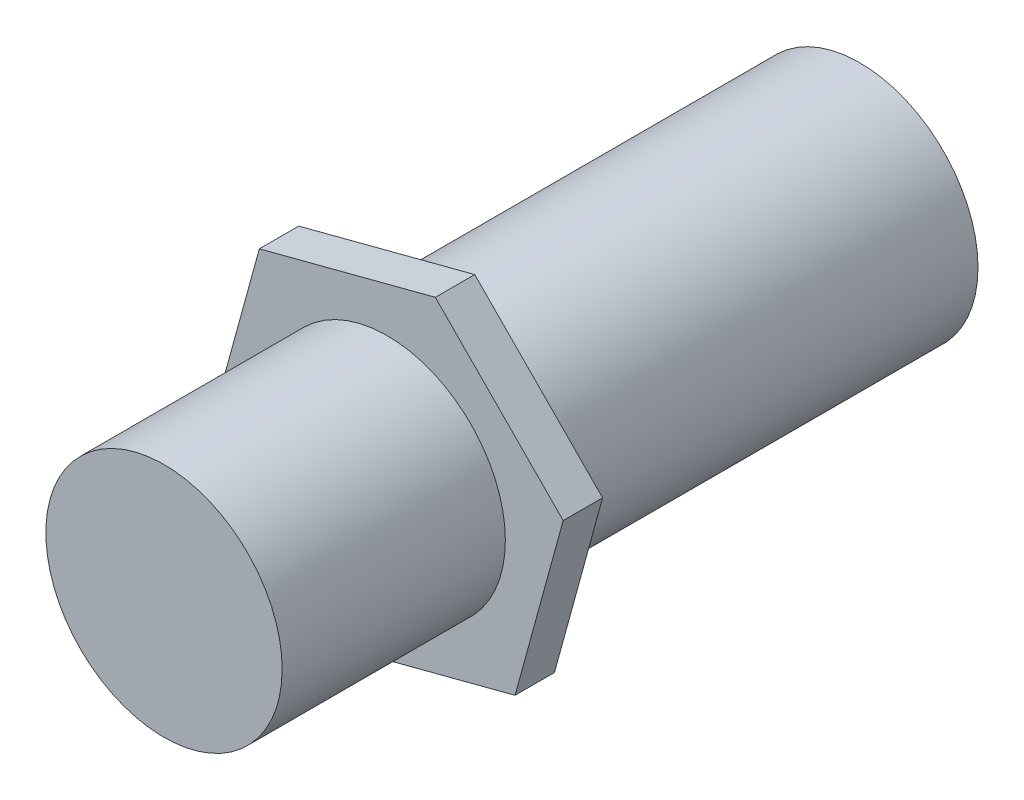
from build123d import *

# Parameters (mm, degrees)
BOSS_EXTRUDE1_DEPTH      = 20
BOSS_EXTRUDE1_DEPTH_BACK = 33
SKETCH1_R                = 9
BOSS_EXTRUDE2_DEPTH      = 3


with BuildPart() as part:
    # Sketch1 → Boss-Extrude1 (new, two sides: drawn at the far end of the back side and taken through both)
    with BuildSketch(Plane.XY.offset(-BOSS_EXTRUDE1_DEPTH_BACK)):
        Circle(SKETCH1_R)
    extrude(amount=BOSS_EXTRUDE1_DEPTH + BOSS_EXTRUDE1_DEPTH_BACK)

    # Sketch2 → Boss-Extrude2 (add)
    with BuildSketch(Plane.XY):
        Polygon((9.738398553, -9.857159511), (13.405749822, 3.505120784), (3.667351269, 13.362280294), (-9.738398553, 9.857159511), (-13.405749822, -3.505120784), (-3.667351269, -13.362280294), align=None)
    extrude(amount=BOSS_EXTRUDE2_DEPTH)


solid = part.part
